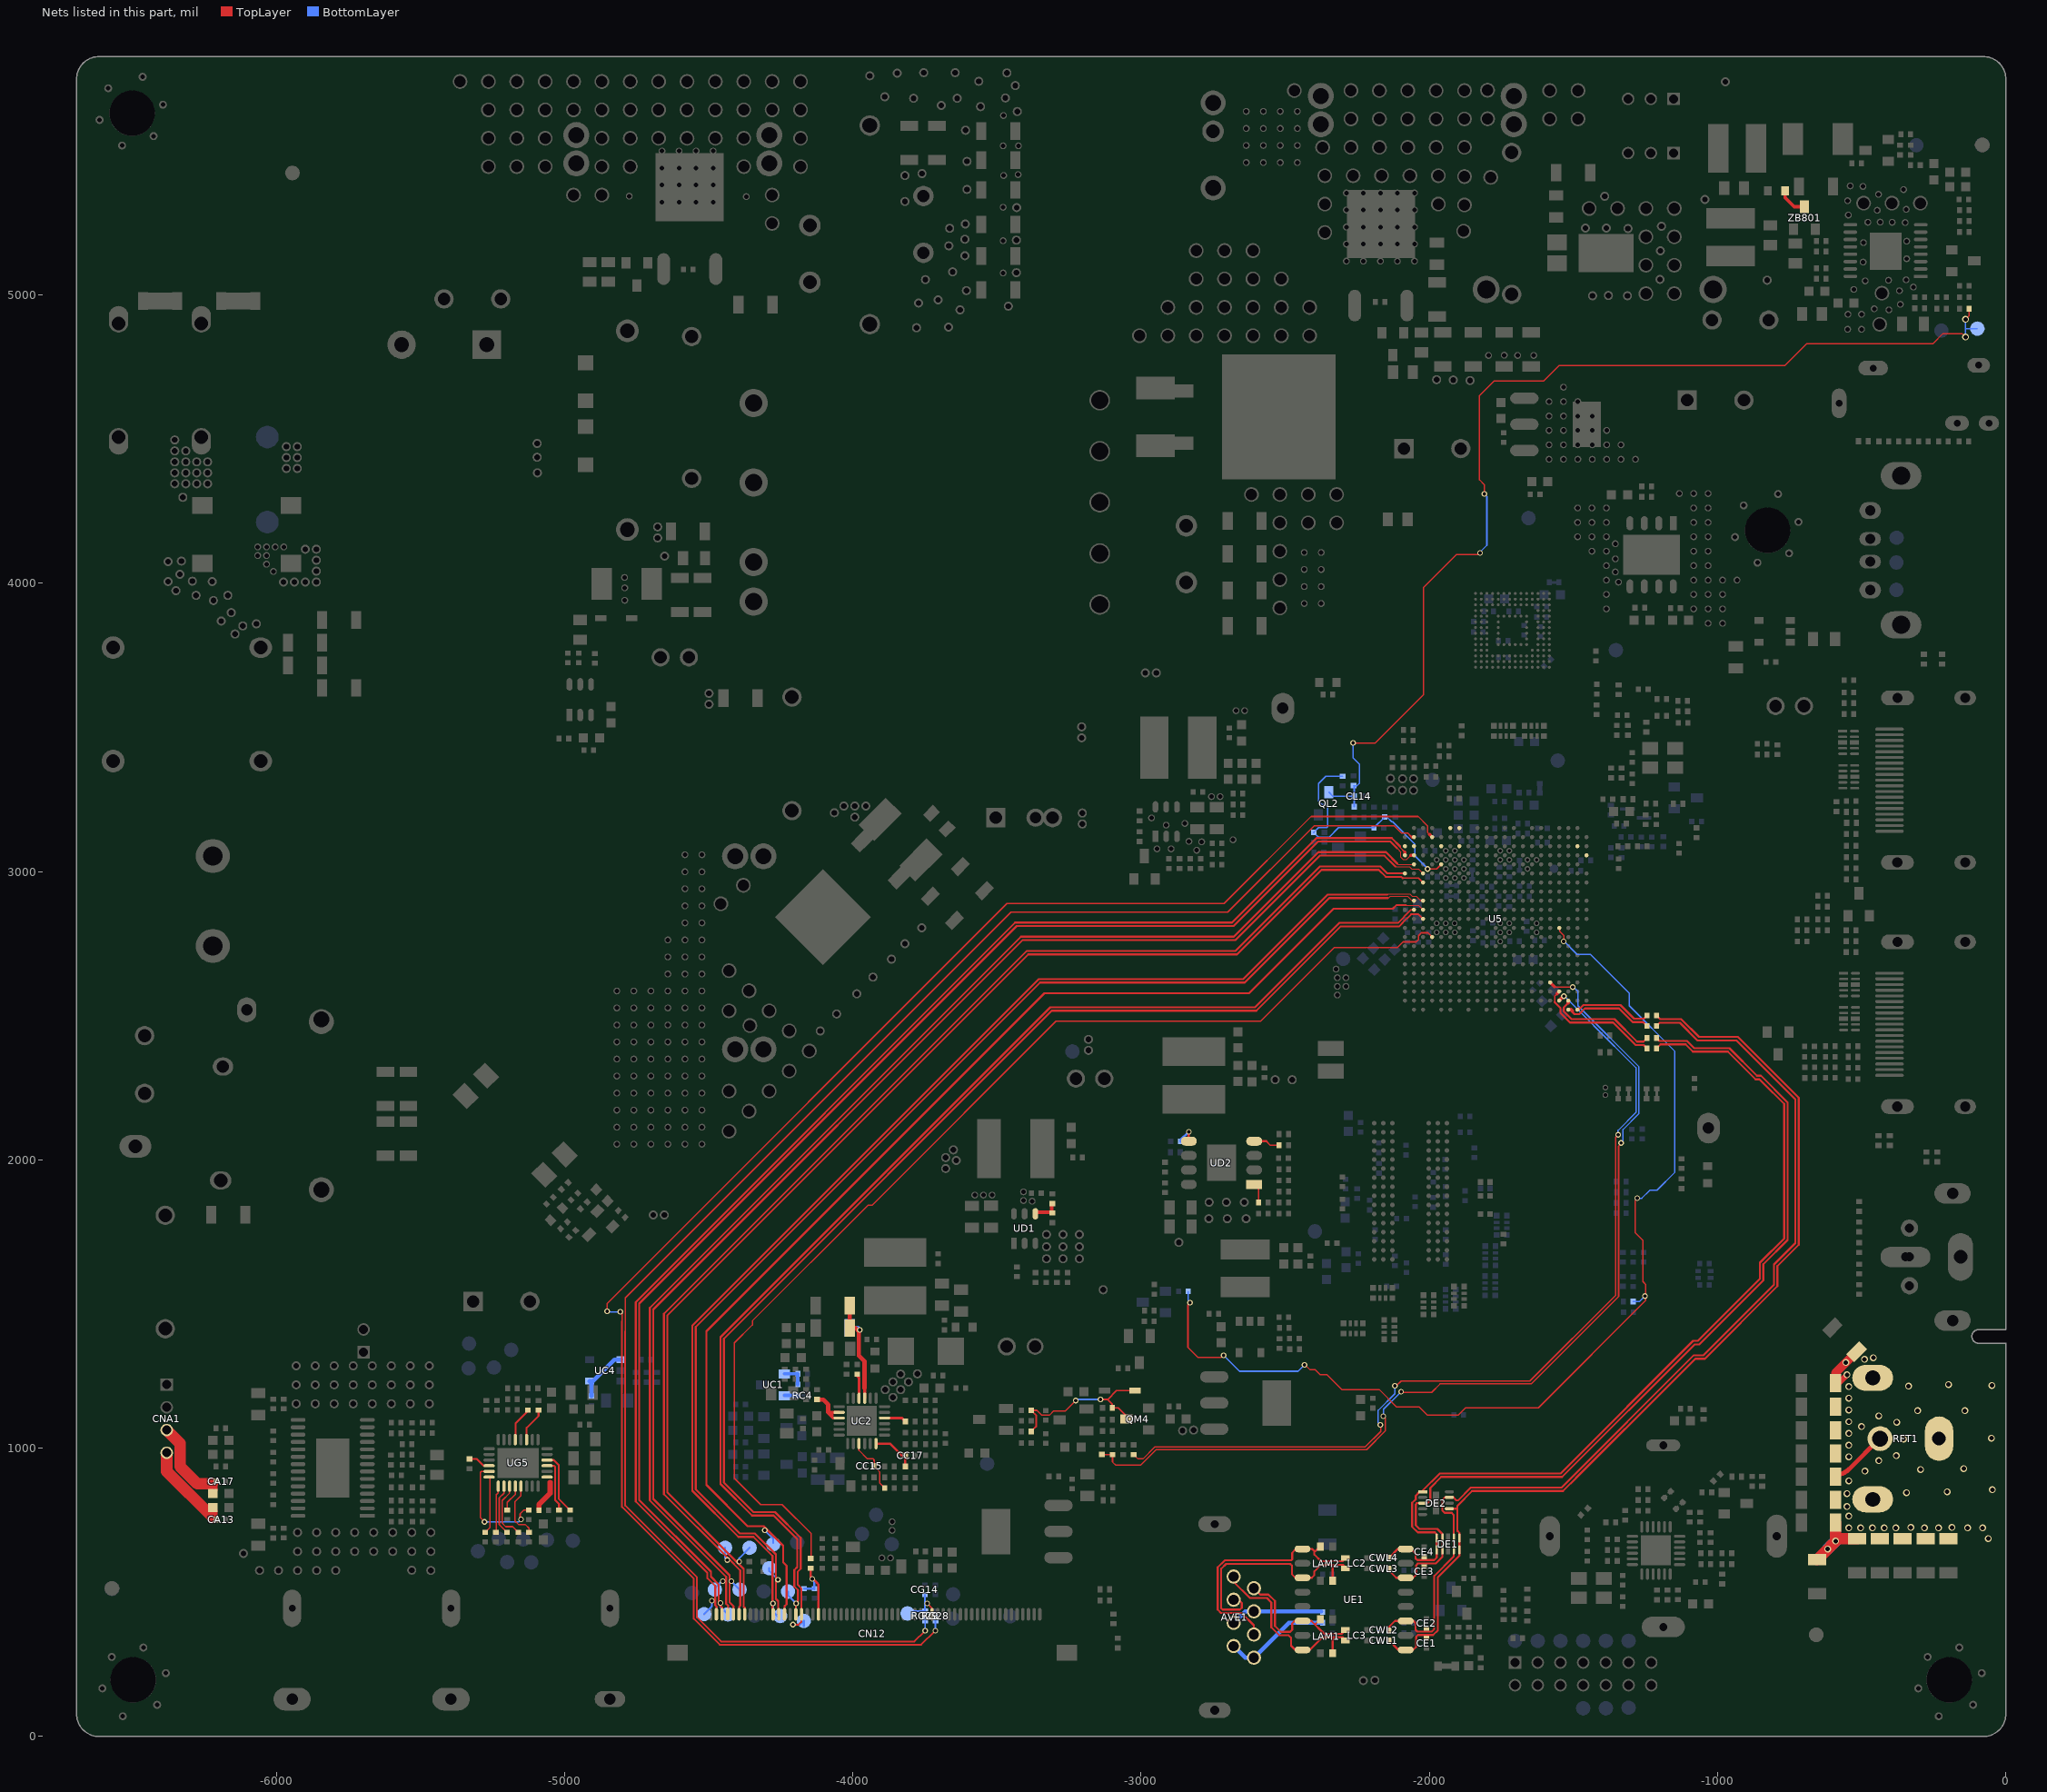
[diagram p0: the nets of this part, all layers, seen from the top]
# Altium PCB MISC84395.PcbDoc (part 22 of 26)
Units mil, origin at the board's own origin, x right, y up, seen from the top; angles counter-clockwise.
Board outline 6692.91 x 5826.77 mil, 2 copper layers (TopLayer, BottomLayer), stack 61.855 mil thick; 951 components, 565 nets, 4374 pads, 1804 vias.
Unrouted connection lines stored in the file: 1.

## Via types
v1: diameter 19.68, hole 11.81, TopLayer to BottomLayer, tented both sides, 1262 vias
v2: diameter 23.62, hole 15.75, TopLayer to BottomLayer, tented both sides, 524 vias
v3: diameter 31.5, hole 19.68, TopLayer to BottomLayer, tented both sides, 11 vias
v4: diameter 24, hole 16, TopLayer to BottomLayer, tented both sides, 6 vias
v5: diameter 19, hole 11.81, TopLayer to BottomLayer, tented both sides, 1 vias

## Nets (pads, with @x,y where several pads share a name; then routed paths per layer and width w, separated by ;. In a path a pad name is that pad's centre, name@x,y a point inside that pad or via, vN(x,y) a via of type N, cw(c..) or ccw(c..) an arc to the next point about the centre after c; other vN are vias at no path point) (continued)
NetRB806_2: RB806.2 ZB801.2 | length 103.8
  TopLayer w11.81: RB806.2@-766.22,5361 -766.22,5337.44 -734.81,5306.03 ZB801.2@-699,5306.03
NetRC2_1: RC2.1 RC3.2 UC1.1 | length 83.8
  BottomLayer w12: UC1.1@-4237.47,1258 RC3.2@-4190.7,1258 RC2.1@-4190.7,1221
NetRC4_1: RC4.1 UC1.2 | length 39.5
  BottomLayer w12: UC1.2@-4237.47,1183 RC4.1@-4198,1183
NetRC8_2: RC8.2 UC2.2 UC2.3 | length 163
  TopLayer w10: -4085.5,1125.04 -4084.91,1124.45 UC2.2@-4047.48,1124.45 ; -4078.11,1117.65 -4078.11,1114.11 -4068.76,1104.76 UC2.3@-4047.48,1104.76
  TopLayer w15: RC8.2@-4124,1168.27 -4102.77,1168.27 -4085.5,1151 -4085.5,1125.04 ; -4084.91,1124.45 -4078.11,1117.65 -4074.23,1113.77
NetRC13_1: RC13.1 UC2.16 | length 77.1
  TopLayer w10: UC2.16@-3890,1104.76 -3829.5,1104.76 RC13.1@-3817.73,1093
NetRC36_1: RC36.1 UC4.1 UC4.4 | length 183.7
  BottomLayer w15: UC4.4@-4913.13,1232.33 -4901.67,1232.33 -4826.87,1307.13 UC4.1@-4804.87,1307.13 ; RC36.1@-4906.73,1181.45 UC4.4@-4906.73,1225.93
NetRD2_2: RD2.2 RD9.2 UD1.4 | length 85.6
  TopLayer w12: UD1.4@-3361.05,1818.73 RD9.2@-3310,1818.73 ; RD9.2@-3310,1815.73 RD2.2@-3310,1850.27
NetRD6_2: RD6.2 UD2.1 | length 69.3
  TopLayer w6: UD2.1@-2607.61,1915 -2592.46,1899.85 RD6.2@-2592.46,1852
NetRD18_1: RD18.1 UD2.4 | length 91.7
  TopLayer w5: -2566,2065 -2552,2051 RD18.1@-2521.73,2051
  TopLayer w8: UD2.4@-2607.61,2065 -2566,2065
NetRD19_1: RD19.1 UD2.5 | length 92.8
  TopLayer w8: UD2.5@-2844.73,2075.35 UD2.5@-2834.39,2065 -2834.39,2096.61 v1(-2834,2097)
  BottomLayer w8: RD19.1@-2864,2064 -2864,2069 v1@-2835,2098
NetRG1_2: RG1.2 UG5.3@-5131.47,1029.71 | length 130
  TopLayer w7: UG5.3@-5131.47,1029.71 -5131.47,1070.59 -5090,1112.06 RG1.2@-5090,1132.27 -5090,1122
NetRG2_2: RG2.2 UG5.5 | length 114.3
  TopLayer w7: UG5.5@-5169.87,1035.71 -5169.87,1086.19 -5127,1129.06 RG2.2@-5127,1132.27
NetRG3_2: RG3.2 UG5.12 | length 78.4
  TopLayer w7: RG3.2@-5330,962.73 -5304.73,962.73 -5281.16,939.16 UG5.12@-5261.39,939.16
NetRG5_2: RG5.2 UG5.23 | length 113.1
  TopLayer w18: RG5.2@-5088.73,785 -5088.73,805.27 -5049.92,844.08 -5049.92,882
NetRG6_1: RG6.1 UC2.22 | length 80.3
  TopLayer w10: RG6.1@-3985,1251.27 -3978.58,1244.85 UC2.22@-3978.58,1173.66
NetRG7_1: RG7.1 RG8.1 RG9.1 UC2.21 | length 401.5
  TopLayer w10: UC2.21@-3958.9,1173.66 -3958.9,1218.1
  TopLayer w15: RG8.1@-4011,1416.76 RG8.1@-4010.94,1416.76 ; RG7.1@-4010.94,1494.76 RG8.1@-4010.94,1416.76 ; -3959.5,1209 -3959.5,1301.61 -3978.78,1320.89 -3978.78,1405.22 -3990.33,1416.76 RG8.1@-4010.94,1416.76
  BottomLayer w15: RG9.1@-4010.94,1417 -3983,1417 v1(-3976,1410)
NetRG79_2: RG79.2 UG5.18 | length 94.2
  TopLayer w5: RG79.2@-5199,785.73 -5199,812 -5170.84,840.16 UG5.18@-5170.84,868.29
NetRG80_2: RG80.2 UG5.19 | length 208.3
  TopLayer w5: UG5.19@-5151.16,868.29 -5151.16,835.84 -5172,815 -5172,748.01 -5158.59,734.59 -5135.18,734.59 -5123.26,722.67 RG80.2@-5123.26,708.73 RG80.2@-5123.26,714.96
NetRG81_2: RG81.2 UG5.13 | length 396.9
  TopLayer w5: v1@-5276.34,744.84 -5277.34,745.84 v1(-5277.34,744.84) -5292,759.5 -5292,916 -5288.53,919.47 UG5.13@-5261.39,919.47 ; v1(-5151,753) -5154,756 -5154,773 -5141.27,785.73 RG81.2@-5124,785.73
  BottomLayer w5: v1@-5276.34,744.84 -5159.16,744.84 v1(-5151,753)
NetRG82_2: RG82.2 UG5.26 | length 219.9
  TopLayer w7: UG5.26@-5060.61,958.84 -5037.22,958.84 -5020.25,941.87 -5020.42,941.7 -5020.42,825.15 RG82.2@-4981,785.73
NetRG84_2: RG84.2 UG5.25 | length 184.8
  TopLayer w7: UG5.25@-5060.61,939.16 -5036.41,939.16 -5032.42,935.17 -5032.42,820.18 -5019,806.76 RG84.2@-5019,785.73
NetRG85_1: RG85.1 UG5.17 | length 207.8
  TopLayer w5: UG5.17@-5190.53,868.29 -5190.53,844.47 -5216.34,818.66 -5216.34,740.3 -5204.04,728 -5180.28,728 RG85.1@-5160.51,708.24
NetRG87_1: RG87.1 UG5.16 | length 177.8
  TopLayer w5: UG5.16@-5210.21,868.29 -5210.21,843.79 -5226.34,827.66 -5226.34,735.07 RG87.1@-5199.51,708.24
NetRG89_1: RG89.1 UG5.15 | length 163.6
  TopLayer w5: RG89.1@-5238.51,708.24 -5236.34,710.41 -5236.34,838.66 -5229.9,845.1 UG5.15@-5229.9,868.29
NetRG91_1: RG91.1 UG5.14 | length 199.4
  TopLayer w5: RG91.1@-5277.93,710.65 RG91.1@-5275.51,708.24 -5259,724.75 UG5.14@-5259,897.39
NX_ADJ_IC: RL1.1 RL3.1 RL7.2 RL10.1 U5.U17 | length 899
  TopLayer w5: v1(-2006.19,3009.31) -1974.69,3009.31 U5.U17@-1958.94,3025.06
  BottomLayer w5: RL1.1@-2401,3135.73 -2384.64,3152.09 -2355.91,3152.09 -2352.25,3155.75 -2352.25,3202 ; RL1.1@-2392.87,3127.6 -2384.64,3119.37 -2347.63,3119.37 -2315,3152 RL7.2@-2191.73,3152 -2155,3188.73 RL10.1@-2155,3189.27 -2147.58,3189.27 -2130.95,3172.64 -2127.41,3172.64 -2050,3095.23 -2050,3054.67 v1@-2006.19,3010.85 ; -2352.25,3210 -2352.25,3202 ; RL3.1@-2301,3330.73 -2359.19,3330.73 -2384.75,3305.18 -2384.75,3244.89 -2373.05,3233.18 -2362.92,3233.18 -2352.25,3222.52 -2352.25,3202
PAIRMODE: CN12.21 RG17.2 RG24.2 RG30.1 | length 234.5
  TopLayer w8: RG17.2@-4146,584.27 -4146,554 -4124.02,532.02 -4119.01,527.01 CN12.21@-4119.01,423.98
  BottomLayer w8: RG30.1@-4168.73,512.73 RG24.2@-4133,512.73 ; RG24.2@-4133,511.73 RG24.2@-4133,512.73 ; -4133,539 RG24.2@-4133,512.73
  other v1: -4141,547
PAIRMODE/: RG17.1 U5.J18 | length 3935.4
  TopLayer w5: RG17.1@-4144.66,619.07 -4144.66,704.22 -4245.07,804.63 -4319.63,804.63 -4411,896 -4411,1365.09 -4348.43,1427.66 -4348.43,1441.8 -3947.89,1842.33 -3933.75,1842.33 -3295.09,2481 -2585.25,2481 -2329.24,2737.01 -2110.14,2737.01 -2090.97,2756.18 -2056.72,2756.18 ; -2053.43,2756.18 -2056.72,2756.18 ; U5.J18@-1990.44,2773.09 -2005.03,2787.68 -2027.98,2787.68 -2038,2777.66 -2038,2764 -2045.82,2756.18 -2056.72,2756.18
PANEL_EN_IC: RM8.1 U5.B4 | length 3178.1
  TopLayer w5: RM8.1@-3026,978.27 -3010.73,963 -2993.76,963 -2951.76,1005 -2221.83,1005 -2168.92,1057.92 -2168.92,1079.92 v1(-2170,1081) ; v1(-2119.87,1216.39) -2114.61,1216.39 -2098,1233 -1675,1233 -1651.33,1233 -1353.17,1531.16 -1353.17,2079.57 v1@-1345.29,2087.46
  TopLayer w12: U5.B4@-1549.5,2552.62 v1@-1533.75,2568.37
  BottomLayer w5: v1(-2170,1081) -2177.34,1088.34 -2177.34,1131.52 -2119.87,1188.99 v1(-2119.87,1216.39) ; v1@-1532.56,2569.07 -1428.95,2465.46 ; -1429.23,2465.18 -1283.49,2319.44 -1283.49,2164 -1345.29,2102.2 v1(-1345.29,2087.01)
  other v1: -1533.51,2568.13
PANEL_ID_DET0_IC: U5.AA15
PANEL_ID_DET1_IC: U5.W15
PANEL_ID_DET2_IC: U5.AA16
PANEL_ON: DM1.A QM4.C RM2.2 RM12.1 RM15.1 | length 594.8
  TopLayer w5: -3362,1131 -3360.58,1131 -3343.95,1114.37 -3318.05,1114.37 -3303.71,1128.72 -3263.28,1128.72 v1(-3227,1165)
  TopLayer w6: RM15.1@-3381.27,1058 -3364.41,1074.85 -3364.41,1114.15 RM2.2@-3381.27,1131 -3362,1131 ; v1(-3141,1169) -3116.32,1169 ; QM4.C@-3046.03,1106.5 -3079.53,1140 RM12.1@-3100.27,1140 -3100.27,1152.94 -3116.32,1169 ; DM1.A@-3020.85,1198.68 DM1.A@-3020.85,1200 -3085.32,1200 -3116.32,1169
  BottomLayer w6: v1(-3227,1165) -3223,1169 v1(-3141,1169)
PC/AV1_LIN_IC: U5.V1
PC/AV1_RIN_IC: U5.W2
PHY_RX_N: CE4.2 CWL4.1 DE1.1 DE1.8 DE2.1 RE14.2 UE1.8 | length 3168.6
  TopLayer w7: CWL4.1@-2140.27,620 -2109.55,650.71 UE1.8@-2081.96,650.71 -2063.71,650.71 -2048,635 -2048,618 -2042,612 -1983,612 -1974.37,620.63 DE1.8@-1974.37,688.47 ; DE1.8@-1974,700.72 -1981.28,708 -2039.97,708 -2059.51,727.54 -2059.51,810.46 -2047.51,822.46 -2047.51,835.12 -2033.63,849 DE2.1@-2023.26,849 -2023.26,852.87 -1963.63,912.5 -1544.7,912.5 -1084.99,1372.21 -1068.63,1372.21 -853.5,1587.34 -853.5,1643.2 -769.5,1727.2 -769.5,2194.28 -842.11,2266.89 -854.94,2279.73 -868.64,2279.73 -964.34,2375.42 -1085.93,2375.42 -1111.32,2400.82 -1197.91,2400.82 RE14.2@-1211.91,2386.82
PHY_RX_N_IC: RE14.1 U5.C4 | length 440.2
  TopLayer w5: -1565.25,2548.27 -1565.25,2568.36 -1557.25,2576.36
  TopLayer w7: -1565.25,2548.27 -1565.25,2546.33 -1545.59,2526.67 -1545.59,2509.7 -1511.92,2476.03 -1362.39,2476.03 -1284.77,2398.41 -1256.98,2398.41 RE14.1@-1245.38,2386.82
  TopLayer w12: -1557.25,2576.36 U5.C4@-1549.5,2584.12
PHY_RX_P: CE3.2 CWL3.1 DE1.2 DE1.7 DE2.3 RE13.2 UE1.6 | length 3260.2
  TopLayer w7: CWL3.1@-2137,583 -2137,573.06 -2114.65,550.71 UE1.6@-2081.96,550.71 -2056.29,550.71 -2045.91,561.09 -2045.91,594.09 -2040,600 -1978.03,600 -1954.68,623.34 -1954.68,702.68 -1972,720 -2035,720 -2047.51,732.51 -2047.51,805.49 -2043.37,809.63 DE2.3@-2023.26,809.63 -2006.37,809.63 -1997,819 -1997,862.16 -1958.66,900.5 -1539.73,900.5 -1080.73,1359.5 -1064.37,1359.5 -841.5,1582.37 -841.5,1638.23 -757.5,1722.23 -757.5,2199.25 -849.97,2291.73 -863.67,2291.73 -959.37,2387.42 -990.73,2387.42 -1080.96,2387.42 -1106.35,2412.82 -1201.91,2412.82 RE13.2@-1211.91,2422.82
PHY_RX_P_IC: RE13.1 U5.B3 | length 380.9
  TopLayer w7: -1518,2544.75 -1533.59,2529.16 -1533.59,2514.67 -1506.95,2488.03 -1357.42,2488.03 -1279.8,2410.41 -1257.78,2410.41 RE13.1@-1245.38,2422.82
  TopLayer w12: -1518,2544.75 U5.B3@-1518,2552.62
PHY_TX_N: CE2.2 CWL2.1 DE1.3 DE1.6 DE2.9 RE12.2 UE1.3 | length 3453.6
  TopLayer w7: CWL2.1@-2140.27,369 -2140.27,379.73 -2119.29,400.71 UE1.3@-2081.96,400.71 -2054.71,400.71 -2048,394 -2048,370 -2042,364 -1991.97,364 -1983,372.97 -1983,556.85 -1915.31,624.53 -1915.31,768.31 -1922.94,775.94 -1946.78,775.94 -1954.99,784.15 -1954.99,820.01 -1945.68,829.32 DE2.9@-1930.74,829.32 -1916.32,829.32 -1906,819 -1900.97,819 -1856.47,863.5 -1541.38,863.5 -1082.38,1322.5 -1049.04,1322.5 -804.5,1567.04 -804.5,1637.05 -730.5,1711.05 -730.5,2210.44 -934.49,2414.42 -1069.77,2414.42 -1131.17,2475.82 -1200.91,2475.82 RE12.2@-1211.91,2464.82
PHY_TX_N_IC: RE12.1 U5.A3 | length 316.6
  TopLayer w7: -1506.36,2515.16 -1496.74,2505.54 -1480.05,2505.54 -1460.55,2525.03 -1342.1,2525.03 -1294.88,2477.82 -1258.38,2477.82 RE12.1@-1245.38,2464.82 RE12.1@-1248.8,2464.82
  TopLayer w12: U5.A3@-1518,2521.12 -1508.79,2521.12 -1504.59,2516.92
PHY_TX_P: CE1.2 CWL1.1 DE1.4 DE1.5 DE2.7 RE11.2 UE1.1 | length 3450.3
  TopLayer w7: CWL1.1@-2140,333 -2107.71,300.71 UE1.1@-2081.96,300.71 -2056.29,300.71 -2045.91,311.09 -2045.91,346.09 -2040,352 -1987,352 -1971,368 -1971,551.88 -1895.63,627.25 DE1.5@-1895.63,688.47 -1895.63,706.32 -1903.31,714 -1903.31,799.69 -1851.5,851.5 -1536.4,851.5 -1488.1,899.81 ; DE2.7@-1930.74,789.95 -1904.26,789.95 ; -1491.45,896.45 -1147.45,1240.45 -1077.4,1310.5 -1044.07,1310.5 -792.5,1562.07 -792.5,1632.08 -718.5,1706.08 -718.5,2215.41 -929.52,2426.42 -1064.8,2426.42 -1126.19,2487.82 -1198.91,2487.82 RE11.2@-1211.91,2500.82
PHY_TX_P_IC: RE11.1 U5.A2 | length 272.6
  TopLayer w7: U5.A2@-1483.2,2521.12 -1481.43,2521.12 -1465.52,2537.03 -1337.13,2537.03 -1289.91,2489.82 -1256.38,2489.82 RE11.1@-1245.38,2500.82
  TopLayer w12: U5.A2@-1486.5,2521.12 -1484.97,2521.12 U5.A2@-1483.2,2522.89
PIN4&5: AVE1.4 AVE1.5 RE3.2 | length 320.4
  BottomLayer w15: AVE1.5@-2678.74,394.09 -2638.58,434.25 AVE1.4@-2608.66,434.25 RE3.2@-2374.98,434.25
PIN7&8: AVE1.7 AVE1.8 RE4.2 | length 372.9
  BottomLayer w15: AVE1.7@-2678.74,313.78 -2638.58,273.62 AVE1.8@-2608.66,273.62 -2487.28,395 RE4.2@-2372.73,395
POL: CG14.2 CN12.41 POL.1 RG29.2 RG29.3 | length 159.7
  TopLayer w6: v1(-3742,462) -3725.31,445.31 CN12.41@-3725.31,423.98
  BottomLayer w6: POL.1@-3796,427 -3788.27,434.73 RG29.2@-3749,434.73 ; RG29.2@-3750,435.73 v1@-3750,462 ; CG14.2@-3750,492.26 v1@-3750,462 ; v1(-3742,462) v1@-3750,462
POWER_DETECT: R27.1 R28.2 U5.D5 | length 3427.1
  TopLayer w5: R28.2@-3136,978.54 -3135.73,978.27 R27.1@-3099,978.27 -3099,952 -3089,942 -3000.62,942 -2947.62,995 -2901,995 ; -2943,995 -2901,995 ; v1(-2160,1111) -2152.55,1103.55 -2152.55,1060.14 -2217.69,995 -2901,995 ; v1@-2096,1194 -1992,1194 -1963,1223 -1647.19,1223 -1343.67,1526.52 -1343.67,2048.16 v1@-1334.83,2057 ; -1565.28,2599.9 v1@-1504.11,2599.9
  TopLayer w10: U5.D5@-1580.99,2615.61 -1565.28,2599.9
  BottomLayer w5: v1@-2159,1112 -2159,1135 v1(-2098,1196) ; v1@-1501.3,2600.81 -1484.91,2584.42 -1484.91,2535 -1273.99,2324.09 -1273.99,2159.35 -1327.95,2105.4 v1@-1327.95,2065.89
  other v1: -1334.83,2059 -1502.49,2599.62
PWM_DIM: CL14.2 PWM_DIM.1 QL2.C RB801.1 RL2.1 RL5.1 | length 3857.4
  TopLayer w5: v1@-2265,3443 v1(-2265,3446) -2187.6,3446 -2112.26,3521.34 -2020.38,3613.22 -2020.38,3985.36 -1929.87,4075.87 ; -1914.87,4090.87 -1929.87,4075.87 ; v1@-1827,4105 -1833.08,4098.92 -1906.82,4098.92 -1929.87,4075.87 ; v1(-1809,4310) -1809,4341.72 -1826,4358.72 -1826,4650.86 -1775.86,4701 -1624,4701 ; -1607,4701 -1624,4701 ; v2(-140,4854) -152,4866 -218.14,4866 -253.14,4831 -691.43,4831 -767.93,4754.5 -1550.5,4754.5 -1604,4701 -1624,4701 ; v2(-140,4915) -127.54,4927.46 RB801.1@-127.54,4952.32
  BottomLayer w5: QL2.C@-2348.5,3275.03 -2334.47,3261 CL14.2@-2260.74,3261 ; v1@-2265.27,3445.73 -2265.27,3394.74 -2242,3371.47 -2242,3307 -2250.99,3298.01 RL2.1@-2263,3298.01 -2260.74,3295.75 CL14.2@-2260.74,3261 ; RL5.1@-2260.73,3225 CL14.2@-2260.73,3261 ; v1@-1827,4105 -1800.55,4131.45 -1800.55,4168 ; v1(-1809,4310) -1800.55,4301.55 -1800.55,4267 ; -1800.55,4136.26 -1800.55,4168 ; -1800.55,4301 -1800.55,4267 ; v2@-140,4864 v2(-140,4915) ; -139,4883 PWM_DIM.1@-99,4883 ; -1800.55,4168 -1800.55,4267
  other v1: -1824,4105
PWR_ON/OFF_IC: RM4.2 RM7.1 U5.K4 | length 3673
  TopLayer w5: -2837.5,1497.5 -2837.5,1349.59 -2802.41,1314.5 -2721.5,1314.5 ; v1@-2431,1289 -2413.82,1271.82 -2395.48,1271.82 -2379.33,1255.66 -2355.73,1255.66 -2303.68,1203.61 -2174.04,1203.61 -2114.03,1143.61 -2035.56,1143.61 -2006.29,1114.34 -1900.86,1114.34 -1874.86,1140.34 -1621.78,1140.34 -1249.66,1512.47 -1249.66,1568.18 -1259.65,1578.17 -1259.65,1720.98 -1286.17,1747.5 -1286.17,1859.77 v1(-1278.83,1867.12) ; U5.K4@-1549.5,2804.59 -1547.9,2802.99 -1547.9,2792.13 -1533.65,2777.87 v1@-1533.65,2757.93
  BottomLayer w5: v1@-2836.54,1511.54 RM7.1@-2836.54,1544 ; v1(-2714,1322) -2659,1267 -2455,1267 v1(-2433,1289) ; v1(-1534.23,2757.34) -1531.97,2757.34 -1487.63,2713.01 -1441.57,2713.01 -1306.3,2577.73 -1306.3,2534.59 -1148.3,2376.59 -1148.3,1957.45 -1210.6,1895.15 -1234.87,1895.15 -1262.9,1867.12 v1(-1278.83,1867.12) ; RM4.2@-1293,1509 -1271.3,1509 v1(-1252.3,1528)
  other v1: -2830,1505
REF: CC17.2 RC22.1 UC2.12 | length 150
  TopLayer w8: UC2.12@-3919.53,1016.18 -3871.83,1016.18 -3830.64,975 CC17.2@-3817.74,975 ; RC22.1@-3817.73,937 CC17.2@-3817.73,968.12
RF: CT60.1 RFT1.1 | length 247.3
  TopLayer w15.8: CT60.1@-590.71,907.55 ccw(c-590.71,970.94) -545.89,926.11 -436.57,1035.43 RFT1.1@-466.9,1005.1
RFGND: CT41.2 CT42.2 CT43.2 CT44.2 CT45.2 CT46.2 CT47.2 CT48.2 CT49.2 CT55.2 CT67.2 CT68.2 CT70.2 RFT1.2 RFT1.3 RFT1.4 | length 493.2
  TopLayer w20: CT48.2@-590.71,1225.55 -580.45,1225.55 v2(-551,1255)
  TopLayer w30: CT48.2@-590.71,1225.55 -590.71,1261.78 CT70.2@-515.21,1337.27
  TopLayer w40: CT45.2@-655.39,613.47 -582.86,686 CT47.2@-516.43,686 ; -607.88,660.98 v2(-590.71,678.15) CT43.2@-590.71,741.55
  BottomLayer w40: v2(-618.31,650.55) -618.31,650.69 -614,655 v2@-589,680
  other v2: -61,687 -503.78,723.71 -463.12,723.71 -422.45,723.71 -381.78,723.71 -545,724 -283,724 -234,724 -133,724 -81,724 -330,725 -187,725 -545,764.67 -551,798 -551,843 -345,846 -204,849 -47,856 -545,886.67 -489,921 -296,926 -146,929 -441,957 -545,970 -380,974 -545,1010.67 -355,1032 -50,1035 -545,1051.33 -501,1075 -379,1090 -545,1092 -441,1112 -306,1130 -142,1130 -545,1132.67 -545,1173.33 -545,1214 -338,1215 -49,1218 -199,1221 -555.62,1296.87 -491,1308 -460,1314
RJ45_FE_RX+: AVE1.3 LAM2.1 LC2.1 UE1.11 | length 845.9
  TopLayer w7: AVE1.3@-2678.74,474.41 -2662.41,474.41 -2651,463 -2651,447 -2657.81,440.19 -2717.21,440.19 -2722,444.97 -2722,582.03 -2705.03,599 -2483,599 -2477,593 -2477,563 -2464.71,550.71 UE1.11@-2440.23,550.71 ; UE1.11@-2427.71,550.71 UE1.11@-2440.23,550.71 ; LAM2.1@-2335.35,540.94 -2335.35,595.35 ; LC2.1@-2280.7,582.95 -2286.95,582.95 -2300,596 -2376,596 -2399,573 -2399,560 -2408.29,550.71 UE1.11@-2440.23,550.71
RJ45_FE_RX-: AVE1.6 LAM2.3 LC2.4 UE1.9 | length 887.6
  TopLayer w7: AVE1.6@-2608.72,354 AVE1.6@-2608.66,353.94 -2608.66,386.04 -2650.81,428.19 -2722.19,428.19 -2734,440 -2734,587 -2710,611 -2480,611 -2476,615 -2476,637 -2462.29,650.71 UE1.9@-2440.23,650.71 -2407,650.71 -2399,642.71 ; LAM2.3@-2387,650.71 LAM2.3@-2378.65,659.06 -2395,642.71 -2399,642.71 ; LC2.4@-2280.7,619.18 -2289.82,619.18 -2301,608 -2376,608 -2399,631 -2399,642.71
RJ45_FE_TX+: AVE1.1 LAM1.1 LC3.1 UE1.16 | length 663.9
  TopLayer w7: AVE1.1@-2678.74,554.72 -2678.74,536.43 -2622.78,480.48 -2563.45,480.48 -2548,465.03 -2548,379.03 -2519.97,351 -2488,351 -2480,343 -2480,315 -2465.71,300.71 UE1.16@-2440.23,300.71 -2414.29,300.71 -2371,344 -2299.75,344 LC3.1@-2288.7,332.95 ; -2335.35,343.65 LAM1.1@-2335.35,288.94 LAM1.1@-2328.7,288.94 ; LC3.1@-2291.95,332.95 LC3.1@-2288.7,332.95 ; LC3.1@-2284.7,332.95 LC3.1@-2288.7,332.95
RJ45_FE_TX-: AVE1.2 LAM1.3 LC3.4 UE1.14 | length 513.7
  TopLayer w7: AVE1.2@-2608.66,514.57 -2586.57,492.48 -2558.48,492.48 -2536,470 -2536,384 -2515,363 -2483,363 -2476,370 -2476,392 -2467.29,400.71 UE1.14@-2440.23,400.71 -2409.71,400.71 -2365,356 -2304,356 -2290.82,369.18 LC3.4@-2284.7,369.18 ; -2395.71,390 LAM1.3@-2378.65,407.06
ROUT+: CA13.2 CNA1.4 LBA1.2 | length 319.7
  TopLayer w12: CA13.2@-6208.75,752.06 LBA1.2@-6208.75,782.98
  TopLayer w40: CNA1.4@-6380,984.25 -6380,919.36 -6222.85,762.21 -6221.5,762.21 -6221.29,762
ROUT-: CA17.1 CNA1.3 LBA2.2 | length 312.9
  TopLayer w12: LBA2.2@-6208.75,854.14 CA17.1@-6208.75,885.16
  TopLayer w40: CNA1.3@-6380,1062.99 -6333.35,1016.34 -6333.35,936.35 -6274,877 -6222,877
RST: CC15.2 RC10.1 UC2.9 | length 202.7
  TopLayer w5: UC2.9@-3978.58,1016.18 -3978.58,992.58 -3949,963 -3929,963 -3926.27,960.26 -3926.27,937 -3906.09,916.82 -3906.09,878.36 RC10.1@-3889.73,862
RXE0N/MLV0N: CN12.17 MLV0N.1 U5.M20 | length 4203.1
  TopLayer w5: -2108.55,2821.4 -2088.38,2841.56 -2088.38,2843.5 -2064.3,2867.58 U5.M20@-2053.43,2867.58
  TopLayer w7: CN12.17@-4196,425.74 CN12.17@-4197.75,423.98 -4197.75,462.31 -4190.07,470 -4190.07,508.34 -4202.76,521.03 -4202.76,577.3 -4192.66,587.4 -4192.66,684.34 -4274.95,766.63 -4349.51,766.63 -4459,876.12 -4459,1384.97 -3314.97,2529 -2605.13,2529 -2312.03,2822.1 -2252.15,2822.1 -2109.25,2822.1
  BottomLayer w7: MLV0N.1@-4225,503 -4225,490 v1(-4197,462)
RXE0P/MLV0P: CN12.18 MLV0P.1 U5.L19 | length 4282.3
  TopLayer w6: -2092.8,2822.3 -2063.26,2851.83 -2037.68,2851.83 U5.L19@-2021.94,2836.08
  TopLayer w7: v1(-4208,388) -4189,388 -4178.07,398.93 CN12.18@-4178.07,423.98 -4178.07,513.31 -4190.76,526 -4190.76,572.33 -4180.66,582.43 -4180.66,689.31 -4269.98,778.63 -4344.54,778.63 -4447,881.09 -4447,1380 -3310,2517 -2600.16,2517 -2307.06,2810.1 -2104.28,2810.1 -2092.44,2821.94
  BottomLayer w7: v1(-4208,388) -4183.34,388 MLV0P.1@-4170,401.34 MLV0P.1@-4170,383
RXE1N: U5.W21
RXE1P: U5.W20
RXE2N/POL_IC: RG29.1 U5.Y20 | length 5517.7
  TopLayer w5: -4789,1406 -4789,1521.66 -3451.66,2859 -2699.4,2859 -2399.58,3158.82 -2122.18,3158.82 -2097.49,3134.14 -2075.79,3134.14 -2062.95,3121.3 -2060.62,3121.3 U5.Y20@-2058.88,3119.55
  TopLayer w6: -4789.5,1406 -4789.5,800.5 -4540.84,551.84 -4540.84,413.24 -4457.11,329.5 -3786.5,329.5 v1(-3749,367)
  TopLayer w12: U5.Y20@-2058.88,3119.55 U5.Y20@-2053.43,3119.55
  BottomLayer w6: v1(-3749,367) RG29.1@-3749,401.27
RXE3P/TP: RG28.1 U5.Y18 | length 5791.8
  TopLayer w5: v1(-4852.5,1475) -4852.5,1501.64 -4837.32,1516.82 ; -4845.05,1509.09 -3465.14,2889 -2712.14,2889 -2410.14,3191 -2038.83,3191 -2006.65,3158.82 -2006.65,3135.75 -1999.47,3128.58 ; v1(-4806.5,1473) -4800.5,1467 -4800.5,1440.5
  TopLayer w6: -4800.5,1440.5 -4800.5,795.94 -4551.84,547.28 -4551.84,408.68 -4461.66,318.5 -3762.5,318.5 v1(-3714,367)
  TopLayer w12: -1999.47,3128.58 U5.Y18@-1990.44,3119.55
  BottomLayer w5: v1(-4852.5,1475) -4850.5,1473 v1(-4806.5,1473) v1@-4807.5,1474
  BottomLayer w6: v1(-3714,367) -3713,368 RG28.1@-3713,401.27 RG28.1@-3713,400
RXE4N/CPV1: U5.W17
RXO0N/MLV5N: CN12.3 MLV5N.1 U5.V21 | length 4640
  TopLayer w5: -2101.51,3087.24 -2101.51,3084.01 -2084.93,3067.42
  TopLayer w6: U5.V21@-2086.08,3056.08 -2085.4,3056.08 U5.V21@-2084.93,3056.56
  TopLayer w7: v1(-4489,471) -4481,471 -4477,475 ; -4477,462 -4477,455.4 -4472.3,450.7 -4472.3,425.03 CN12.3@-4473.35,423.98 ; -4477,464 -4477,475 ; CN12.3@-4475,419.73 CN12.3@-4473.35,418.08 ; -2101.51,3087.24 -2130.37,3116.1 -2391.38,3116.1 -2684.48,2823 -3436.75,2823 -4753,1506.75 -4753,815.61 -4504.34,566.96 -4504.34,549.37 -4477,522.03 -4477,475
  TopLayer w10: U5.V21@-2084.93,3056.56 -2084.93,3067.42
  BottomLayer w7: MLV5N.1@-4515.72,424.49 -4489,451.21 v1(-4489,471)
RXO0P/MLV5P: CN12.4 MLV5P.1 U5.V20 | length 4639
  TopLayer w3.94: -2112.51,3081.27 -2098.98,3067.74 -2098.98,3050.73 -2090.75,3042.5 -2079.11,3042.5 -2065.05,3056.56
  TopLayer w7: CN12.4@-4453.66,423.98 -4453.66,447.66 -4460.3,454.3 -4460.3,455.67 -4465,460.37 -4465,527 -4492.34,554.34 -4492.34,571.93 -4741,820.58 -4741,1501.78 -3431.78,2811 -2679.51,2811 -2386.41,3104.1 -2135.34,3104.1 -2112.51,3081.27
  TopLayer w10: -2065.05,3056.56 U5.V20@-2053.43,3056.56
  BottomLayer w7: v1(-4458.66,463) -4458.66,449.66 MLV5P.1@-4433,424
RXO1N/MLV4N: CN12.5 MLV4N.1 U5.U20 | length 4551.5
  TopLayer w3.94: -2110.79,3027.65 -2108.2,3025.06 U5.U20@-2053.43,3025.06
  TopLayer w7: v1(-4451,539) -4439.34,539 ; CN12.5@-4433.98,423.98 -4432.46,425.5 -4432.46,453.54 -4439.34,460.43 -4439.34,539 ; -2111.01,3027.44 -2150.67,3067.1 -2385.23,3067.1 -2678.33,2774 -3416.45,2774 -4704,1486.45 -4704,818.94 -4439.34,554.28 -4439.34,539
  BottomLayer w7: MLV4N.1@-4478.28,509.48 -4478.28,514.72 v1@-4452.5,540.5
RXO1P/MLV4P: CN12.6 MLV4P.1 U5.T19 | length 4556.8
  TopLayer w3.94: -2118.19,3017.19 -2069.18,3017.19 -2061.31,3009.31 -2037.68,3009.31 U5.T19@-2021.94,2993.56
  TopLayer w7: CN12.6@-4414.29,423.98 -4414.29,452.35 -4427.34,465.4 -4427.34,559.25 -4692,823.91 -4692,1481.48 -3411.48,2762 -2701.64,2762 -2673.36,2762 -2380.26,3055.1 -2155.64,3055.1 -2117.96,3017.42
  BottomLayer w7: v1@-4419,536 MLV4P.1@-4393,510
  other v1: -4421,539
RXO2N/MLV3N: CN12.7 MLV3N.1 U5.T21 | length 4425.5
  TopLayer w6: U5.T21@-2086.95,2995.58 -2085.15,2993.79 U5.T21@-2084.93,2993.56
  TopLayer w7: CN12.7@-4394.61,423.98 -4394,424.59 -4394,450 -4390.34,453.66 -4390.34,576.34 -4430.5,616.5 -4655,841 -4655,1466.15 -3396.15,2725 -2686.32,2725 -2672.18,2725 -2379.07,3018.1 -2170.97,3018.1 -2146.65,2993.79 U5.T21@-2085.15,2993.79
  BottomLayer w7: MLV3N.1@-4443,655 -4443,620 v1(-4435,612)
RXO2P/MLV3P: CN12.8 MLV3P.1 U5.R19 | length 4490.3
  TopLayer w5: -2093.2,2977.82 -2037.68,2977.82 U5.R19@-2021.94,2962.07
  TopLayer w7: CN12.8@-4374.92,423.98 -4374.92,446.6 -4378.34,450.02 -4378.34,581.31 -4399.01,601.99 -4643,845.97 -4643,1461.18 -3391.18,2713 -2667.21,2713 -2374.1,3006.1 -2177.28,3006.1 -2176.61,3006.78 -2151.62,2981.79 -2097.17,2981.79 -2093.2,2977.82
  BottomLayer w7: v1(-4394,607) -4394,618.76 MLV3P.1@-4358.28,654.48
RXO3N/MLV2N: CN12.13 MLV2N.1 U5.N19 | length 4363.9
  TopLayer w3.94: -2147.12,2920.43 -2144.85,2922.7 -2067.21,2922.7 -2059.34,2914.82 -2045.56,2914.82 -2029.81,2899.08 U5.N19@-2021.94,2899.08
  TopLayer w7: CN12.13@-4276.49,423.98 -4276.49,432.49 -4278.66,434.66 -4278.66,626.6 -4344.69,692.63 -4397.13,692.63 -4557,852.5 -4557,1425.56 -3355.56,2627 -2645.73,2627 -2352.62,2920.1 -2211.56,2920.1 -2146.8,2920.1
  BottomLayer w7: v1(-4277,462) -4277,433 MLV2N.1@-4262,418
RXO3P/MLV2P: CN12.14 MLV2P.1 U5.N20 | length 4324.8
  TopLayer w3.94: -2143.37,2906.78 -2135.33,2914.82 -2075.09,2914.82 -2059.34,2899.08 U5.N20@-2053.43,2899.08
  TopLayer w7: v1(-4260,544) v1@-4266.66,550.66 ; CN12.14@-4256.81,423.98 -4258.66,425.83 -4258.66,469.6 -4266.66,477.6 -4266.66,544 v1@-4266.66,550.66 ; -2144.69,2908.1 -2216.53,2908.1 -2347.65,2908.1 -2640.76,2615 -3350.59,2615 -4545,1420.59 -4545,857.47 -4392.16,704.63 -4339.72,704.63 -4266.66,631.57 v1@-4266.66,550.66
  BottomLayer w7: MLV2P.1@-4290,584 -4290,574 v1(-4260,544)
RXO4N/MLV1N: CN12.15 MLV1N.1 U5.M19 | length 4291.9
  TopLayer w3.94: -2081.63,2883.33 -2037.68,2883.33 U5.M19@-2021.94,2867.58
  TopLayer w7: CN12.15@-4237.12,423.98 -4237.12,451.88 -4229.66,459.34 -4229.66,592.69 -4241.66,604.69 -4241.66,661.69 -4309.6,729.63 -4364.84,729.63 -4508,872.79 -4508,1405.26 -3335.26,2578 -2625.43,2578 -2332.33,2871.1 -2231.86,2871.1 -2126.72,2871.1 -2114.5,2883.33 -2081.63,2883.33
  BottomLayer w7: v1(-4305,715) -4276,686 MLV1N.1@-4276,672